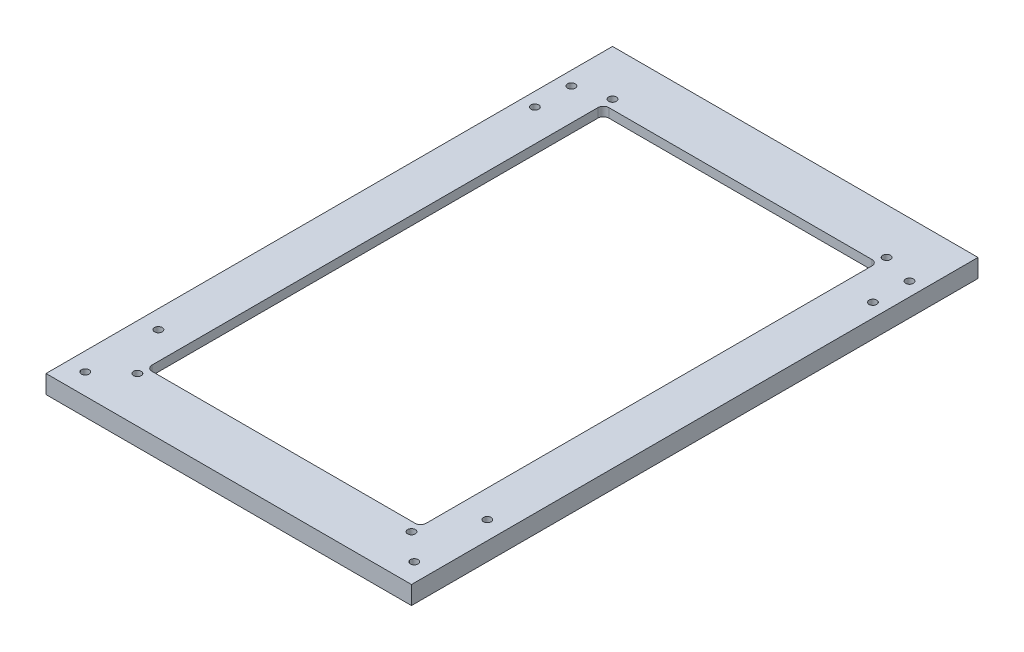
SolidWorks part; units mm, degrees
material "6061"
ref_plane "前视基准面" through (0, 0, 0) normal (0, 0, 1) x (1, 0, 0)
ref_plane "上视基准面" through (0, 0, 0) normal (0, 1, 0) x (1, 0, 0)
ref_plane "右视基准面" through (0, 0, 0) normal (1, 0, 0) x (0, 0, -1)
sketch "草图1" plane through (0, 0, 0) normal (0, 1, 0) x (1, 0, 0)
  line L1 (100, -155) -> (-100, -155)
  line L2 (100, -155) -> (100, 155)
  line L3 (100, 155) -> (-100, 155)
  line L4 (-100, -155) -> (-100, 155)
  line L5 (100, -155) -> (-100, 155) construction
  line L6 (100, 155) -> (-100, -155) construction
  point P0 (0, 0)
  dimension "D1" = 200
  dimension "D2" = 310
extrude "凸台-拉伸1" add sketch "草图1" along normal mid plane 10
sketch "草图2" plane through (0, -5, 0) normal (0, -1, 0) x (1, 0, 0)
  line L1 (-75, -125) -> (75, -125)
  line L2 (-75, -125) -> (-75, 125)
  line L3 (-75, 125) -> (75, 125)
  line L4 (75, -125) -> (75, 125)
  line L5 (-75, -125) -> (75, 125) construction
  line L6 (-75, 125) -> (75, -125) construction
  point P0 (0, 0)
  dimension "D1" = 150
  dimension "D2" = 250
extrude "切除-拉伸1" cut sketch "草图2" against normal through all
fillet "圆角1" radius 3 4 edges at (-75, 0, 125) (75, 0, 125) (75, 0, -125) (-75, 0, -125)
sketch "草图13" plane through (0, -5, 0) normal (0, -1, 0) x (1, 0, 0)
  line L1 (-85, 140) -> (85, 140)
  line L2 (-85, 140) -> (-85, -140)
  line L3 (-85, -140) -> (85, -140)
  line L4 (85, 140) -> (85, -140)
  line L5 (-85, 140) -> (85, -140) construction
  line L6 (-85, -140) -> (85, 140) construction
  point P0 (0, 0)
  dimension "D1" = 170
  dimension "D2" = 280
extrude "切除-拉伸2" cut sketch "草图13" against normal blind 5
hole_wizard "M5 螺纹孔4" positions "草图14" profile "草图15" tap size "M5" standard "GB" end condition up to next
sketch "草图14" plane through (0, 5, 0) normal (0, 1, 0) x (1, 0, 0)
  point P0 (92.5, 105)
  point P3 (92.5, 125)
  point P6 (-92.5, 105)
  point P9 (-92.5, 125)
sketch "草图15" plane through (92.5, 5, -105) normal (1, 0, 0) x (0, 0, 1)
  line L0 (0, 0) -> (0, 10)
  line L1 (0, 10) -> (2.1, 10)
  line L2 (2.1, 10) -> (2.1, 0)
  line L5 (2.1, 0) -> (0, 0)
  line L11 (0, -6.35) -> (0, 107.95) construction
  dimension "通孔螺纹孔钻头直径" = 4.2
  dimension "通孔螺纹孔钻头深度" = 10
cosmetic thread "孔螺蚊线20" parameters "D2"=5
cosmetic thread "孔螺蚊线21" parameters "D2"=5
cosmetic thread "孔螺蚊线22" parameters "D2"=5
cosmetic thread "孔螺蚊线23" parameters "D2"=5
fillet "圆角2" radius 5 4 edges at (-85, -2.5, -140) (85, -2.5, -140) (85, -2.5, 140) (-85, -2.5, 140)
hole_wizard "M5 螺纹孔5" positions "草图16" profile "草图17" tap size "M5" standard "GB" end condition through all
sketch "草图16" plane through (0, 5, 0) normal (0, 1, 0) x (1, 0, 0)
  point P0 (-90, -103.5)
  point P3 (-90, -143.5)
  point P7 (90, -103.5)
  point P10 (90, -143.5)
sketch "草图17" plane through (-90, 5, 103.5) normal (1, 0, 0) x (0, 0, 1)
  line L0 (0, 0) -> (0, 10)
  line L1 (0, 10) -> (2.1, 10)
  line L2 (2.1, 10) -> (2.1, 0)
  line L5 (2.1, 0) -> (0, 0)
  line L11 (0, -6.35) -> (0, 107.95) construction
  dimension "通孔螺纹孔钻头直径" = 4.2
  dimension "通孔螺纹孔钻头深度" = 10
cosmetic thread "孔螺蚊线24" parameters "D2"=5
cosmetic thread "孔螺蚊线25" parameters "D2"=5
cosmetic thread "孔螺蚊线26" parameters "D2"=5
cosmetic thread "孔螺蚊线27" parameters "D2"=5
hole_wizard "M5 螺纹孔6" positions "草图18" profile "草图19" tap size "M5" standard "GB" end condition through all
sketch "草图18" plane through (0, 0, 0) normal (0, -1, 0) x (-1, 0, 0)
  point P0 (75, -130)
  point P3 (-75, -130)
  point P6 (75, 130)
  point P9 (-75, 130)
sketch "草图19" plane through (-75, 0, 130) normal (1, 0, 0) x (0, 0, -1)
  line L0 (0, 0) -> (0, 5)
  line L1 (0, 5) -> (2.1, 5)
  line L2 (2.1, 5) -> (2.1, 0)
  line L5 (2.1, 0) -> (0, 0)
  line L11 (0, -6.35) -> (0, 107.95) construction
  dimension "通孔螺纹孔钻头直径" = 4.2
  dimension "通孔螺纹孔钻头深度" = 5
cosmetic thread "孔螺蚊线28" parameters "D2"=5
cosmetic thread "孔螺蚊线29" parameters "D2"=5
cosmetic thread "孔螺蚊线30" parameters "D2"=5
cosmetic thread "孔螺蚊线31" parameters "D2"=5
